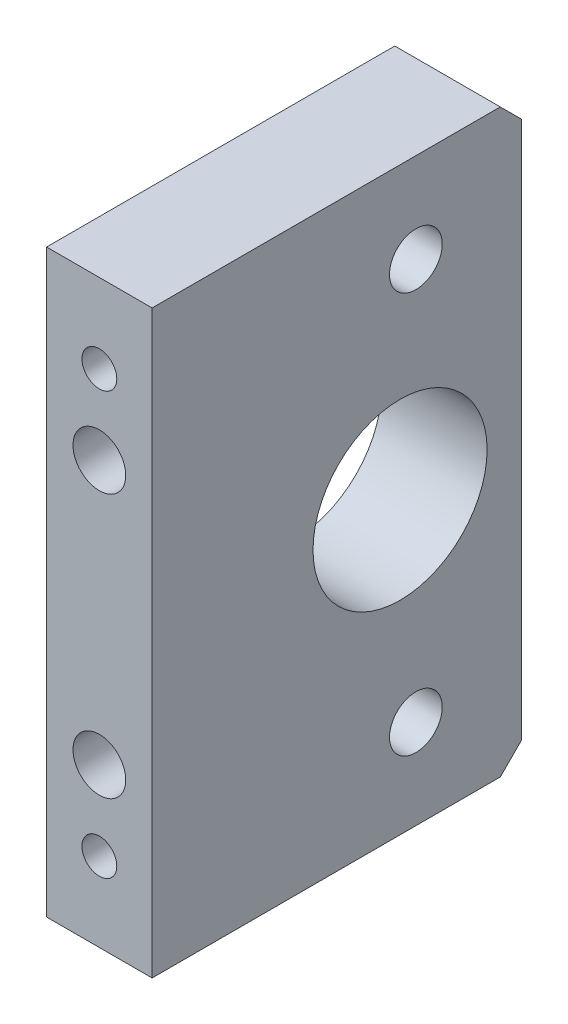
SolidWorks part; units mm, degrees
material "6061铝"
ref_plane "前视基准面" through (0, 0, 0) normal (0, 0, 1) x (1, 0, 0)
ref_plane "上视基准面" through (0, 0, 0) normal (0, 1, 0) x (1, 0, 0)
ref_plane "右视基准面" through (0, 0, 0) normal (1, 0, 0) x (0, 0, -1)
sketch "草图1" plane through (0, 0, 0) normal (1, 0, 0) x (0, 0, -1)
  line L1 (-17.5, 27.5) -> (17.5, 27.5)
  line L2 (-17.5, 27.5) -> (-17.5, -27.5)
  line L3 (-17.5, -27.5) -> (17.5, -27.5)
  line L4 (17.5, 27.5) -> (17.5, -27.5)
  line L5 (-17.5, 27.5) -> (17.5, -27.5) construction
  line L6 (-17.5, -27.5) -> (17.5, 27.5) construction
  point P0 (0, 0)
  dimension "D1" = 35
  dimension "D2" = 55
extrude "凸台-拉伸1" add sketch "草图1" along normal blind 10
sketch "草图2" plane through (0, 0, 0) normal (-1, 0, 0) x (0, 0, 1)
  line L0 (0, 0) -> (-4.8334, 0) construction
  line L1 (-17.5, -27.5) -> (-17.5, 27.5) construction
  circle A0 centre (-6, 0) radius 8.25
  dimension "D1" = 16.5
  dimension "D2" = 11.5
extrude "切除-拉伸1" cut sketch "草图2" against normal blind 110
hole_wizard "M6 螺纹孔1" positions "草图4" profile "草图6" tap size "M6" standard "GB" end condition through all
sketch "草图4" plane through (0, 0, 0) normal (-1, 0, 0) x (0, 0, 1)
  line L1 (17.5, 27.5) -> (17.5, -27.5) construction
  point P0 (-7.5, -19)
  dimension "D1" = 19
  dimension "D2" = 25
sketch "草图6" plane through (0, -19, -7.5) normal (0, 1, 0) x (0, 0, 1)
  line L0 (0, 0) -> (0, 10)
  line L1 (0, 10) -> (2.5, 10)
  line L2 (2.5, 10) -> (2.5, 0)
  line L5 (2.5, 0) -> (0, 0)
  line L11 (0, -6.35) -> (0, 107.95) construction
  dimension "通孔螺纹孔钻头直径" = 5
  dimension "通孔螺纹孔钻头深度" = 10
cosmetic thread "孔螺蚊线1" parameters "D2"=6
mirror "镜向1" about plane through (0, 0, 0) normal (0, 1, 0) of "M6 螺纹孔1"
hole_wizard "M4 螺纹孔1" positions "草图7" profile "草图9" tap size "M4" standard "GB"
sketch "草图7" plane through (0, 0, 17.5) normal (0, 0, 1) x (1, 0, 0)
  line L0 (0, 0) -> (21.0367, 0) construction
  line L2 (0, 27.5) -> (0, -27.5) construction
  point P0 (5, 20)
  point P8 (5, -20)
  dimension "D1" = 5
  dimension "D2" = 40
sketch "草图9" plane through (5, 20, 17.5) normal (1, 0, 0) x (0, -1, 0)
  line L0 (0, 0) -> (0, 11.0914)
  line L1 (0, 11.0914) -> (1.65, 10.1)
  line L2 (1.65, 10.1) -> (1.65, 0)
  line L5 (1.65, 0) -> (0, 0)
  line L10 (0, 11.0914) -> (-1.65, 10.1) construction
  line L11 (0, -6.35) -> (0, 107.95) construction
  dimension "螺纹孔钻头直径" = 3.3
  dimension "螺纹孔钻头深度" = 10.1
  dimension "导头角度" = 118
cosmetic thread "孔螺蚊线2" parameters "D1"=8, "D2"=4
cosmetic thread "孔螺蚊线3" parameters "D1"=8, "D2"=4
hole_wizard "Ø5.0 (5) 直径孔1" positions "草图10" profile "草图11" hole size "Ø5.0" standard "GB"
sketch "草图10" plane through (0, 0, 17.5) normal (0, 0, 1) x (1, 0, 0)
  line L0 (0, 0) -> (21.3791, 0) construction
  line L2 (0, 27.5) -> (0, -27.5) construction
  point P0 (5, 12.5)
  point P2 (5, -12.5)
  dimension "D1" = 5
  dimension "D2" = 25
sketch "草图11" plane through (5, 12.5, 17.5) normal (1, 0, 0) x (0, -1, 0)
  line L0 (0, 0) -> (0, 11.6022)
  line L1 (0, 11.6022) -> (2.5, 10.1)
  line L2 (2.5, 10.1) -> (2.5, 0)
  line L5 (2.5, 0) -> (0, 0)
  line L10 (0, 11.6022) -> (-2.5, 10.1) construction
  line L11 (0, -6.35) -> (0, 107.95) construction
  dimension "孔直径" = 5
  dimension "孔深度" = 10.1
  dimension "导头角度" = 118
chamfer "倒角1" distance 2 angle 45 2 edges at (5, -27.5, -17.5) (5, 27.5, -17.5)
